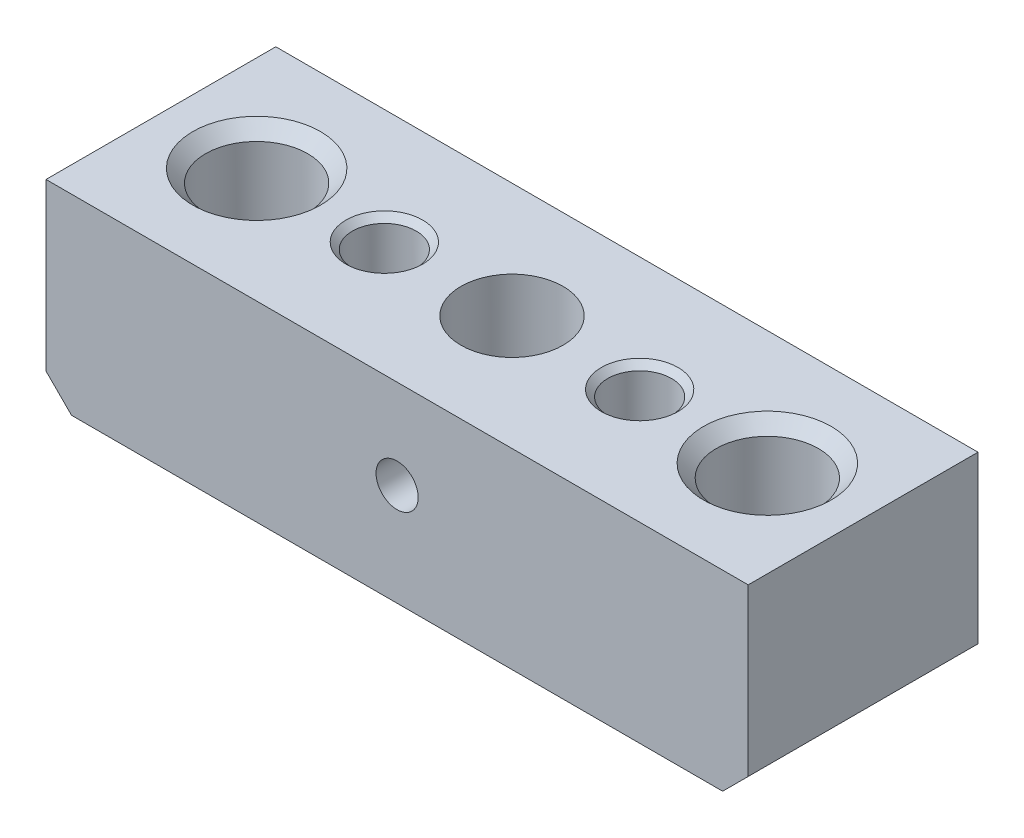
from build123d import *

# Parameters (mm, degrees)
SKETCH1_W                  = 55
SKETCH1_H                  = 18
BOSS_EXTRUDE1_DEPTH        = 30
SKETCH2_R                  = 4
CUT_EXTRUDE1_DEPTH         = 25
SKETCH3_R                  = 2.5
CUT_EXTRUDE2_DEPTH         = 38
SKETCH4_W                  = 75
SKETCH4_H                  = 27
SKETCH4_R                  = 4
BOSS_EXTRUDE2_DEPTH        = 10
BOSS_EXTRUDE3_START        = 10
SKETCH6_W                  = 75
SKETCH6_H                  = 18
SKETCH6_R                  = 4
BOSS_EXTRUDE3_DEPTH        = 10
SKETCH7_W                  = 75
SKETCH7_H                  = 20
CUT_EXTRUDE3_DEPTH         = 31
SKETCH8_R                  = 1.280962141
CUT_EXTRUDE4_DEPTH         = 24
F_8_2_8_2_DIAMETER_HOLE1_D = 8
CHAMFER1_SIZE              = 2
SKETCH10_R                 = 2.5
CUT_EXTRUDE5_DEPTH         = 25
SKETCH11_R                 = 1.362041629
CUT_EXTRUDE6_DEPTH         = 10
M4_TAPPED_HOLE1_D          = 3.3
M4_TAPPED_HOLE1_DEPTH      = 10.1
M4_TAPPED_HOLE1_TIP        = 0.991420021
SKETCH13_W                 = 55
SKETCH13_H                 = 5
CUT_EXTRUDE7_DEPTH         = 22
CHAMFER2_SIZE              = 0.5
CHAMFER3_SIZE              = 1


with BuildPart() as part:
    # Sketch1 → Boss-Extrude1 (new body)
    with BuildSketch(Plane(origin=(0, 0, 0), x_dir=(1, 0, 0), z_dir=(0, 1, 0))):
        Rectangle(SKETCH1_W, SKETCH1_H)
    extrude(amount=BOSS_EXTRUDE1_DEPTH)

    # Sketch2 → Cut-Extrude1 (cut)
    with BuildSketch(Plane(origin=(0, 30, 0), x_dir=(1, 0, 0), z_dir=(0, 1, 0))):
        with Locations(Location((-20, 0, 0), (0, 0, 270))):
            Circle(SKETCH2_R)
        with Locations(Location((20, 0, 0), (0, 0, 90))):
            Circle(SKETCH2_R)
    extrude(amount=-CUT_EXTRUDE1_DEPTH, mode=Mode.SUBTRACT)

    # Sketch3 → Cut-Extrude2 (cut)
    with BuildSketch(Plane(origin=(0, 30, 0), x_dir=(1, 0, 0), z_dir=(0, 1, 0))):
        with Locations(Location((-20, 0, 0), (0, 0, 270))):
            Circle(SKETCH3_R)
        with Locations(Location((20, 0, 0), (0, 0, 270))):
            Circle(SKETCH3_R)
    extrude(amount=-CUT_EXTRUDE2_DEPTH, mode=Mode.SUBTRACT)

    # Sketch4 → Boss-Extrude2 (add)
    with BuildSketch(Plane(origin=(0, 30, 0), x_dir=(1, 0, 0), z_dir=(0, 1, 0))):
        Rectangle(SKETCH4_W, SKETCH4_H)
        with Locations(Location((-20, 0, 0), (0, 0, 270))):
            Circle(SKETCH4_R, mode=Mode.SUBTRACT)
        with Locations(Location((20, 0, 0), (0, 0, 90))):
            Circle(SKETCH4_R, mode=Mode.SUBTRACT)
    extrude(amount=-BOSS_EXTRUDE2_DEPTH)

    # Sketch6 → Boss-Extrude3 (add)
    with BuildSketch(Plane(origin=(0, 30, 0), x_dir=(1, 0, 0), z_dir=(0, 1, 0)).offset(BOSS_EXTRUDE3_START)):
        Rectangle(SKETCH6_W, SKETCH6_H)
        with Locations(Location((-20, 0, 0), (0, 0, 270))):
            Circle(SKETCH6_R, mode=Mode.SUBTRACT)
        with Locations(Location((20, 0, 0), (0, 0, 270))):
            Circle(SKETCH6_R, mode=Mode.SUBTRACT)
    extrude(amount=-BOSS_EXTRUDE3_DEPTH)

    # Sketch7 → Cut-Extrude3 (cut)
    with BuildSketch(Plane.XY.offset(13.5)):
        with Locations((0, 30)):
            Rectangle(SKETCH7_W, SKETCH7_H)
    extrude(amount=-CUT_EXTRUDE3_DEPTH, mode=Mode.SUBTRACT)

    # Sketch8 → Cut-Extrude4 (cut)
    with BuildSketch(Plane(origin=(0, 20, 0), x_dir=(1, 0, 0), z_dir=(0, 1, 0))):
        with Locations(Location((0, 0, 0), (0, 0, 270))):
            Circle(SKETCH8_R)
    extrude(amount=-CUT_EXTRUDE4_DEPTH, mode=Mode.SUBTRACT)

    # Ø8.2 (8.2) Diameter Hole1 (through all)
    with Locations(Plane.ZX.offset(20)):
        with Locations((0, 0)):
            Hole(F_8_2_8_2_DIAMETER_HOLE1_D / 2)

    # Chamfer1
    chamfer1_edges = [part.edges().sort_by_distance(p)[0] for p in [
        (-27.5, 0, 0),
        (27.5, 0, 0),
    ]]
    chamfer(chamfer1_edges, length=CHAMFER1_SIZE)

    # Sketch10 → Cut-Extrude5 (cut)
    with BuildSketch(Plane(origin=(0, 20, 0), x_dir=(1, 0, 0), z_dir=(0, 1, 0))):
        with Locations(Location((-10, 0, 0), (0, 0, 270))):
            Circle(SKETCH10_R)
        with Locations(Location((10, 0, 0), (0, 0, 270))):
            Circle(SKETCH10_R)
    extrude(amount=-CUT_EXTRUDE5_DEPTH, mode=Mode.SUBTRACT)

    # Sketch11 → Cut-Extrude6 (cut)
    with BuildSketch(Plane.XY.offset(9)):
        with Locations((0, 8)):
            Circle(SKETCH11_R)
    extrude(amount=-CUT_EXTRUDE6_DEPTH, mode=Mode.SUBTRACT)

    # M4 Tapped Hole1
    with Locations(Plane(origin=(0, 8, 9), x_dir=(1, 0, 0), z_dir=(0, 0, 1))):
        with Locations((0, 0)):
            Hole(M4_TAPPED_HOLE1_D / 2, depth=M4_TAPPED_HOLE1_DEPTH)
            with Locations((0, 0, -(M4_TAPPED_HOLE1_DEPTH + M4_TAPPED_HOLE1_TIP / 2))):  # 118° drill point
                Cone(0, M4_TAPPED_HOLE1_D / 2, M4_TAPPED_HOLE1_TIP, mode=Mode.SUBTRACT)

    # Sketch13 → Cut-Extrude7 (cut)
    with BuildSketch(Plane.XY.offset(9)):
        with Locations((0, 17.5)):
            Rectangle(SKETCH13_W, SKETCH13_H)
    extrude(amount=-CUT_EXTRUDE7_DEPTH, mode=Mode.SUBTRACT)

    # Chamfer2
    chamfer2_edges = [part.edges().sort_by_distance(p)[0] for p in [
        (-10, 0, -2.5),
        (10, 0, -2.5),
        (10, 15, -2.5),
        (-10, 15, -2.5),
    ]]
    chamfer(chamfer2_edges, length=CHAMFER2_SIZE)

    # Chamfer3
    chamfer3_edges = [part.edges().sort_by_distance(p)[0] for p in [
        (-20, 15, -4),
        (20, 15, 4),
    ]]
    chamfer(chamfer3_edges, length=CHAMFER3_SIZE)


solid = part.part
